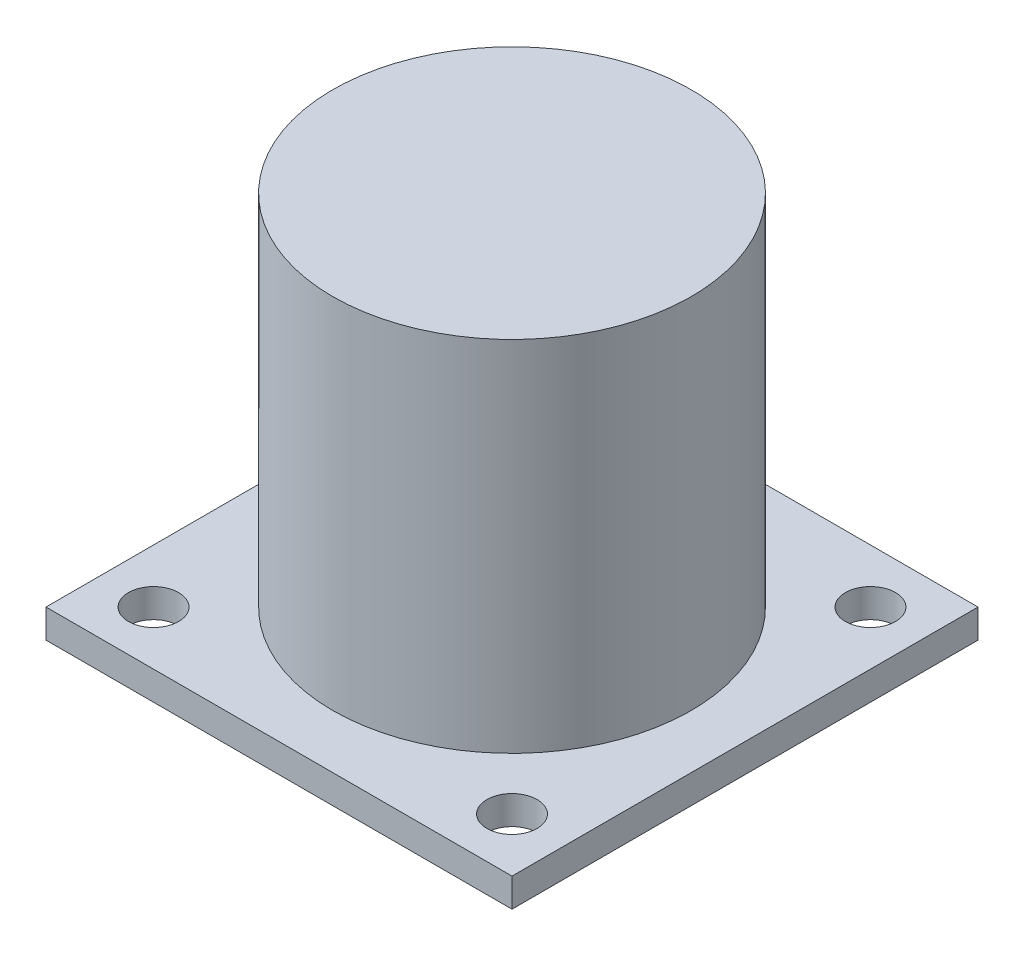
from build123d import *

# Parameters (mm, degrees)
SKETCH1_W                      = 130
SKETCH1_H                      = 130
BOSS_EXTRUDE1_DEPTH            = 8
SKETCH2_R                      = 50
BOSS_EXTRUDE2_DEPTH            = 100
F_14_0_14_DIAMETER_HOLE1_D     = 14
F_14_0_14_DIAMETER_HOLE1_DEPTH = 22
F_14_0_14_DIAMETER_HOLE1_TIP   = 4.206024333


with BuildPart() as part:
    # Sketch1 → Boss-Extrude1 (new body)
    with BuildSketch(Plane(origin=(0, 0, 0), x_dir=(1, 0, 0), z_dir=(0, 1, 0))):
        Rectangle(SKETCH1_W, SKETCH1_H)
    extrude(amount=BOSS_EXTRUDE1_DEPTH)

    # Sketch2 → Boss-Extrude2 (add)
    with BuildSketch(Plane(origin=(0, 8, 0), x_dir=(1, 0, 0), z_dir=(0, 1, 0))):
        with Locations(Location((0, 0, 0), (0, 0, 270))):
            Circle(SKETCH2_R)
    extrude(amount=BOSS_EXTRUDE2_DEPTH)

    # Ø14.0 (14) Diameter Hole1
    with Locations(Plane(origin=(0, 8, 0), x_dir=(1, 0, 0), z_dir=(0, 1, 0))):
        with Locations((-50, 50), (50, 50), (50, -50), (-50, -50)):
            Hole(F_14_0_14_DIAMETER_HOLE1_D / 2, depth=F_14_0_14_DIAMETER_HOLE1_DEPTH)
            with Locations((0, 0, -(F_14_0_14_DIAMETER_HOLE1_DEPTH + F_14_0_14_DIAMETER_HOLE1_TIP / 2))):  # 118° drill point
                Cone(0, F_14_0_14_DIAMETER_HOLE1_D / 2, F_14_0_14_DIAMETER_HOLE1_TIP, mode=Mode.SUBTRACT)


solid = part.part
